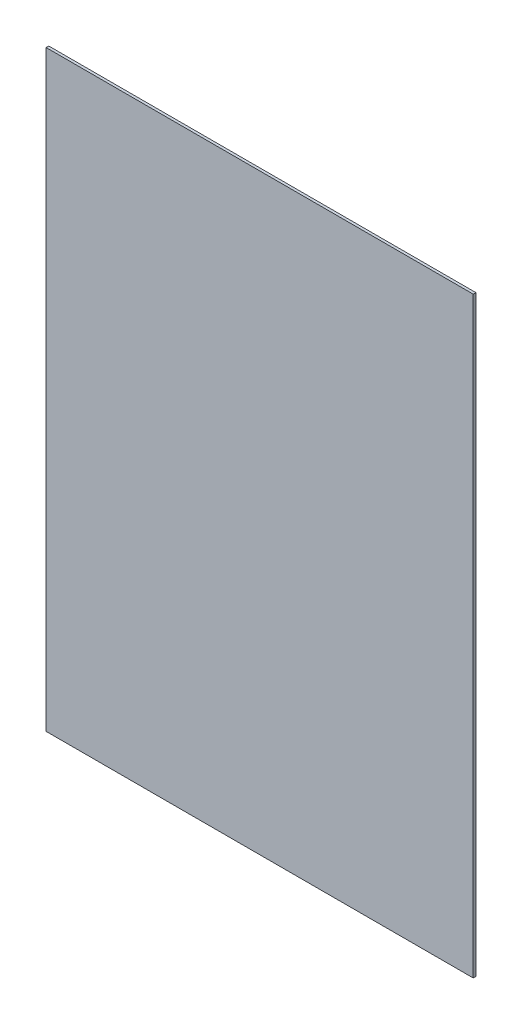
from build123d import *

# Parameters (mm, degrees)
SKETCH_1_W      = 807
SKETCH_1_H      = 1119
EXTRUDE_1_DEPTH = 5


with BuildPart() as part:
    # 草图1 → 凸台-拉伸1 (new body)
    with BuildSketch(Plane.XY):
        Rectangle(SKETCH_1_W, SKETCH_1_H)
    extrude(amount=EXTRUDE_1_DEPTH)


solid = part.part
